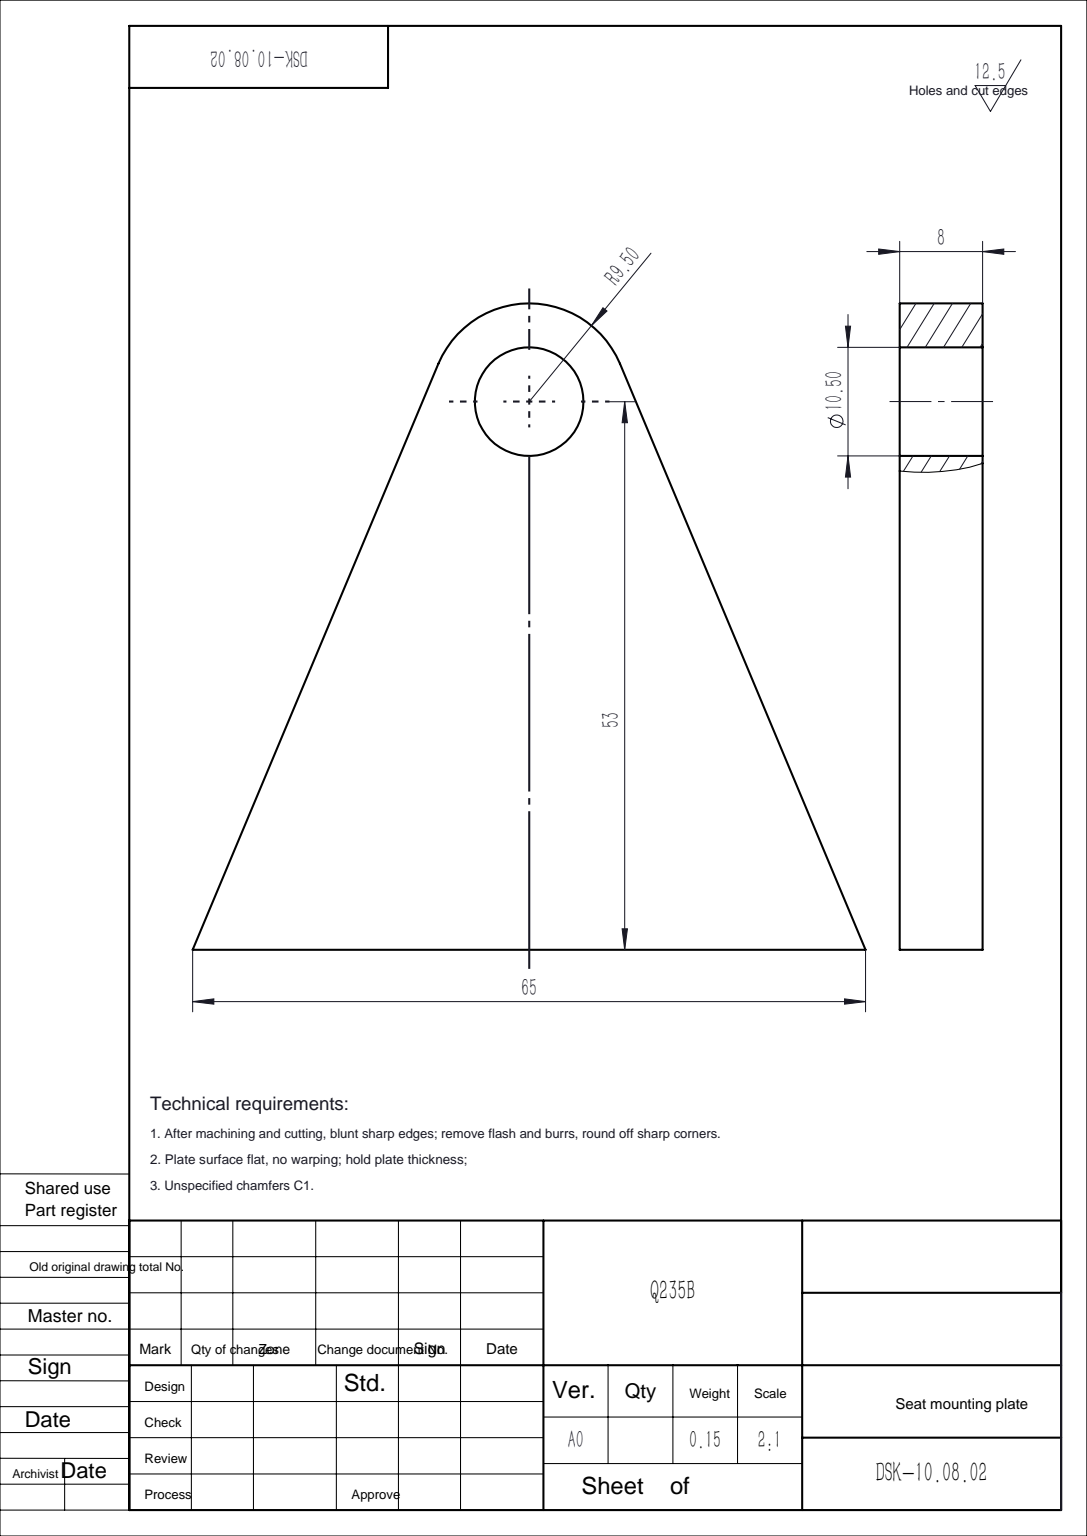
SolidWorks part; units mm, degrees
material "Q235B"
ref_plane "Front Plane" through (0, 0, 0) normal (0, 0, 1) x (1, 0, 0)
ref_plane "Top Plane" through (0, 0, 0) normal (0, 1, 0) x (1, 0, 0)
ref_plane "Right Plane" through (0, 0, 0) normal (1, 0, 0) x (0, 0, -1)
sketch "Sketch1" plane through (0, 0, 0) normal (0, 0, 1) x (1, 0, 0)
  line L0 (-32.5, 0) -> (32.5, 0)
  line L1 (32.5, 0) -> (8.7624, 56.6703)
  line L2 (0, 62.5) -> (0, 0) construction
  line L3 (-32.5, 0) -> (-8.7624, 56.6703)
  arc A0 (8.7624, 56.6703) -> (-8.7624, 56.6703) centre (0, 53) ccw
  circle A1 centre (0, 53) radius 5.25
  dimension "D1" = 53
  dimension "D2" = 9.5
  dimension "D4" = 10.5
  dimension "D3" = 65
extrude "Boss-Extrude1" add sketch "Sketch1" along normal blind 8
